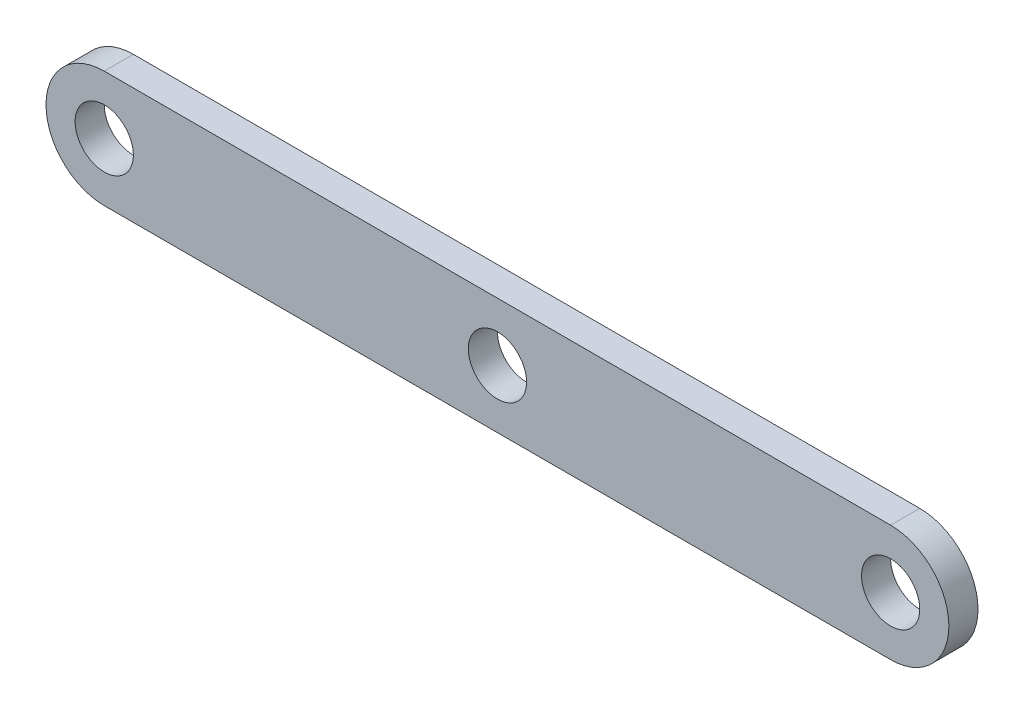
SolidWorks part; units mm, degrees
ref_plane "Front Plane" through (0, 0, 0) normal (0, 0, 1) x (1, 0, 0)
ref_plane "Top Plane" through (0, 0, 0) normal (0, 1, 0) x (1, 0, 0)
ref_plane "Right Plane" through (0, 0, 0) normal (1, 0, 0) x (0, 0, -1)
sketch "Sketch1" plane through (0, 0, 0) normal (0, 0, 1) x (1, 0, 0)
  line L0 (-135, 0) -> (135, 0) construction
  line L1 (-135, 20) -> (135, 20)
  line L2 (-135, -20) -> (135, -20)
  arc A0 (-135, 20) -> (-135, -20) centre (-135, 0) ccw
  arc A1 (135, -20) -> (135, 20) centre (135, 0) ccw
  point P2 (0, 0)
  dimension "D1" = 20
  dimension "D2" = 270
extrude "Boss-Extrude1" add sketch "Sketch1" along normal blind 10
sketch "Sketch2" plane through (0, 0, 10) normal (0, 0, 1) x (1, 0, 0)
  circle A0 centre (-135, 0) radius 10
  circle A1 centre (135, 0) radius 10
  dimension "D1" = 20
extrude "Cut-Extrude1" cut sketch "Sketch2" against normal through all
sketch "Sketch3" plane through (0, 0, 10) normal (0, 0, 1) x (1, 0, 0)
  circle A0 centre (0, 0) radius 10
  circle A1 centre (-135, 0) radius 10 construction
extrude "Cut-Extrude2" cut sketch "Sketch3" against normal blind 10
